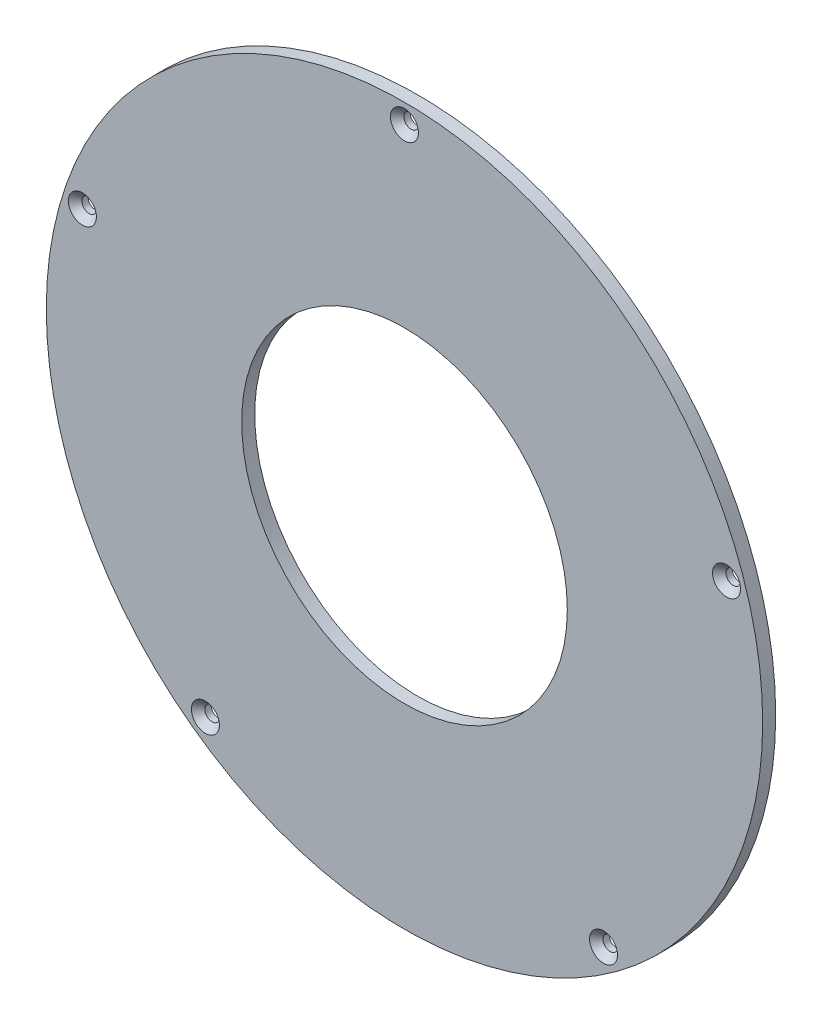
SolidWorks part; units mm, degrees
material "ABS"
ref_plane "Front Plane" through (0, 0, 0) normal (0, 0, 1) x (1, 0, 0)
ref_plane "Top Plane" through (0, 0, 0) normal (0, 1, 0) x (1, 0, 0)
ref_plane "Right Plane" through (0, 0, 0) normal (1, 0, 0) x (0, 0, -1)
sketch "Sketch1" plane through (0, 0, 0) normal (0, 0, 1) x (1, 0, 0)
  circle A0 centre (0, 0) radius 50
  circle A1 centre (0, 0) radius 110
  dimension "D1" = 220
  dimension "D2" = 100
extrude "Boss-Extrude1" add sketch "Sketch1" along normal blind 4
hole_wizard "Hole Size (% per cross) Slotted Countersunk Wood Screw Type1" positions "Sketch4" profile "Sketch5" countersink size "M4" standard "GB" end condition up to next
sketch "Sketch4" plane through (0, 0, 4) normal (0, 0, 1) x (1, 0, 0)
  line L0 (0, 0) -> (0, 104) construction
  line L2 (0, 0) -> (145.2757, 0) construction
  circle A0 centre (0, 0) radius 104 construction
  point P0 (0, 104)
  point P26 (98.9099, 32.1378)
  point P27 (61.1297, -84.1378)
  point P28 (-61.1297, -84.1378)
  point P29 (-98.9099, 32.1378)
  dimension "D1" = 208
  dimension "D2" = 5
sketch "Sketch5" plane through (0, 104, 4) normal (1, 0, 0) x (0, -1, 0)
  line L0 (0, 0) -> (0, 4)
  line L1 (0, 4) -> (2.25, 4)
  line L2 (2.25, 4) -> (2.25, 2.05)
  line L3 (2.25, 2.05) -> (4.3, 0)
  line L5 (4.3, 0) -> (0, 0)
  line L6 (-2.25, 2.05) -> (-4.3, 0) construction
  line L11 (0, -6.35) -> (0, 107.95) construction
  dimension "通孔孔直径" = 4.5
  dimension "通孔孔深度" = 4
  dimension "近端锥形沉头孔直径" = 8.6
  dimension "近端锥形沉头孔角度" = 90
